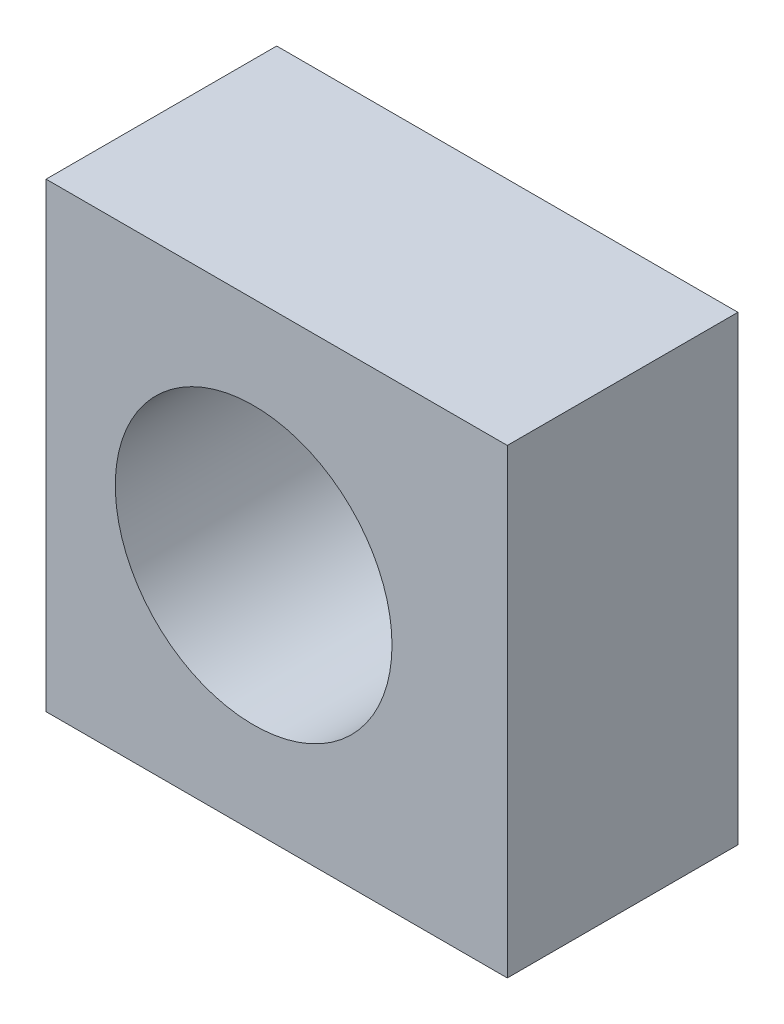
from build123d import *

# Parameters (mm, degrees)
SKETCH1_W           = 20
SKETCH1_H           = 20
SKETCH1_R           = 6
BOSS_EXTRUDE1_DEPTH = 10


with BuildPart() as part:
    # Sketch1 → Boss-Extrude1 (new body)
    with BuildSketch(Plane.XY):
        Rectangle(SKETCH1_W, SKETCH1_H)
        with Locations((-1, 0)):
            Circle(SKETCH1_R, mode=Mode.SUBTRACT)
    extrude(amount=BOSS_EXTRUDE1_DEPTH)


solid = part.part
